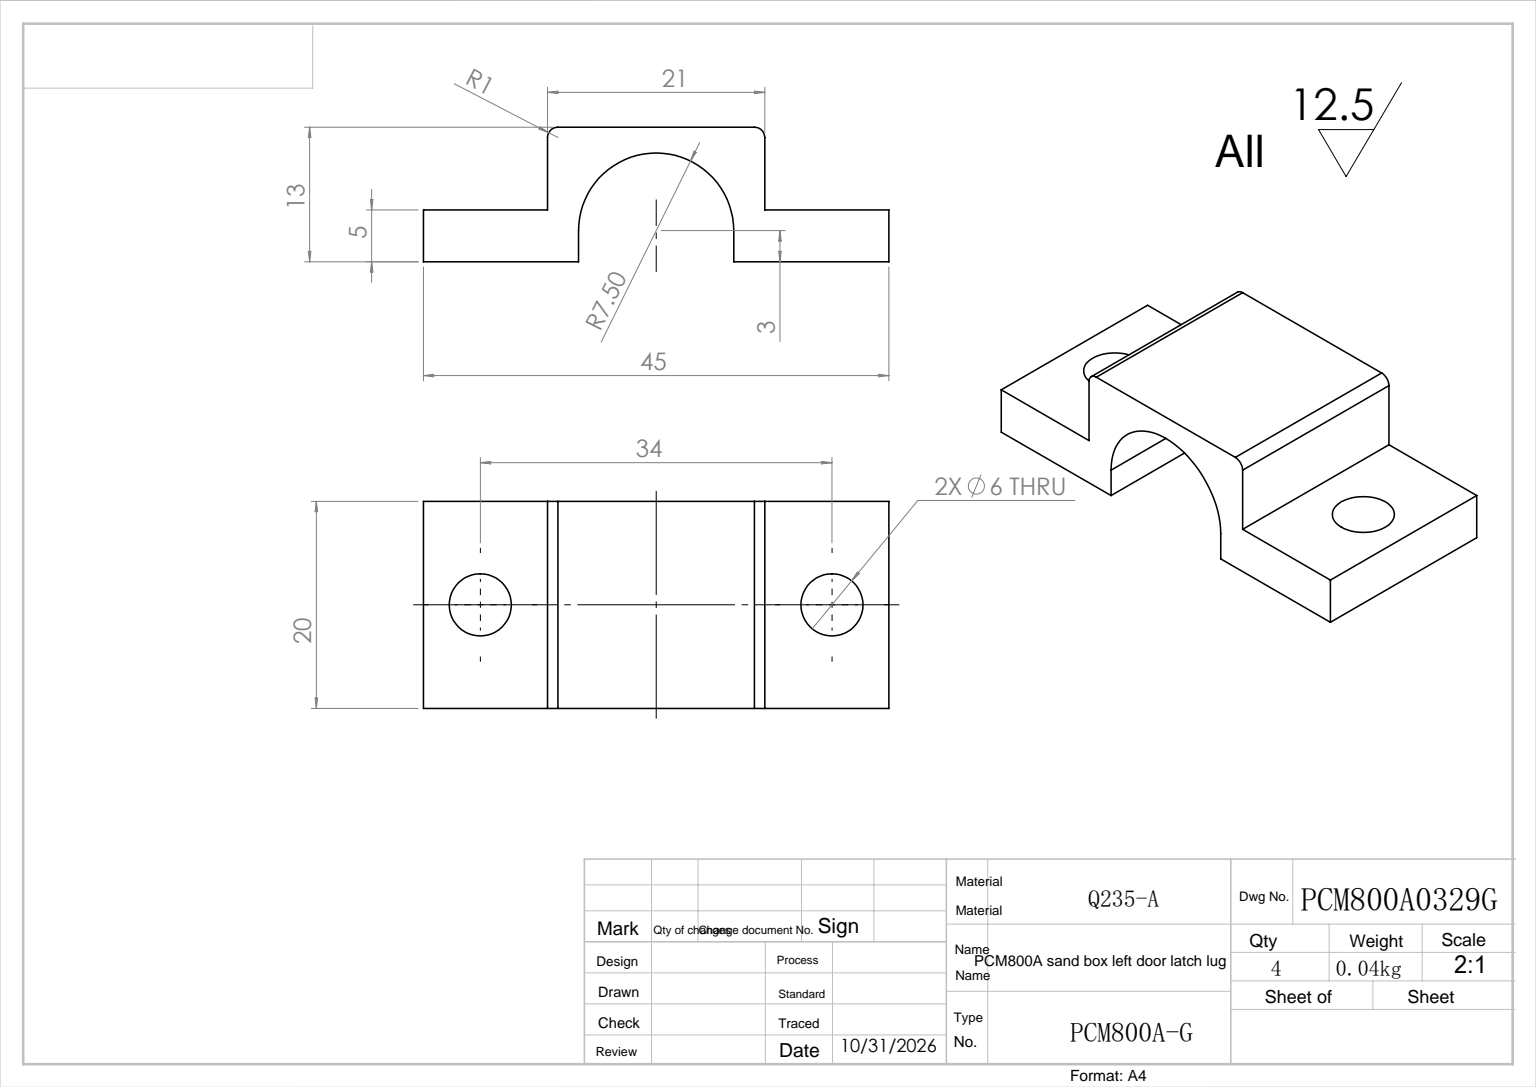
SolidWorks part; units mm, degrees
ref_plane "前视基准面" through (0, 0, 0) normal (0, 0, 1) x (1, 0, 0)
ref_plane "上视基准面" through (0, 0, 0) normal (0, 1, 0) x (1, 0, 0)
ref_plane "右视基准面" through (0, 0, 0) normal (1, 0, 0) x (0, 0, -1)
sketch "草图1" plane through (0, 0, 0) normal (0, 0, 1) x (1, 0, 0)
  line L0 (0, 0) -> (12, 0)
  line L1 (12, 0) -> (12, 8)
  line L2 (12, 8) -> (33, 8)
  line L3 (33, 8) -> (33, 0)
  line L4 (33, 0) -> (45, 0)
  line L5 (45, 0) -> (45, -5)
  line L6 (15, -2) -> (15, -5)
  line L7 (30, -2) -> (30, -5)
  line L8 (15, -5) -> (0, -5)
  line L10 (45, -5) -> (30, -5)
  line L11 (0, -5) -> (0, 0)
  arc A0 (30, -2) -> (15, -2) centre (22.5, -2) ccw
  dimension "D6" = 15
  dimension "D7" = 3
  dimension "D1" = 21
  dimension "D2" = 12
  dimension "D3" = 12
  dimension "D4" = 13
  dimension "D5" = 5
extrude "凸台-拉伸1" add sketch "草图1" along normal blind 20
fillet "圆角1" radius 1 2 edges at (33, 8, 10) (12, 8, 10)
sketch "草图2" plane through (0, 0, 0) normal (0, 1, 0) x (1, 0, 0)
  line L0 (45, -20) -> (45, 0) construction
  circle A0 centre (5.5, -10) radius 3
  circle A1 centre (39.5, -10) radius 3
  dimension "D1" = 6
  dimension "D2" = 5.5
  dimension "D3" = 34
extrude "切除-拉伸1" cut sketch "草图2" against normal through all
